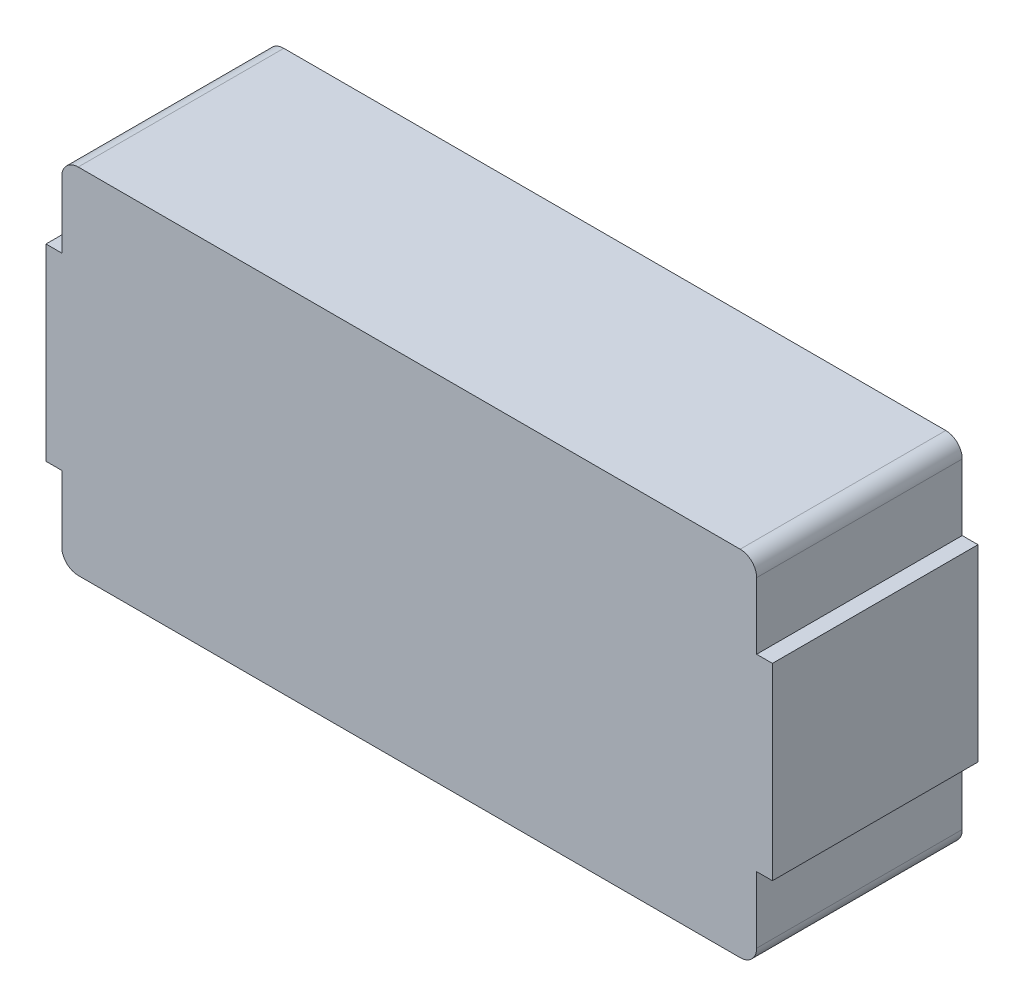
from build123d import *

# Parameters (mm, degrees)
BOSS_EXTRUDE1_DEPTH = 4
BOSS_EXTRUDE2_DEPTH = 25
FILLET1_R           = 2


with BuildPart() as part:
    # Sketch1 → Boss-Extrude1 (new body)
    with BuildSketch(Plane.XY):
        with BuildLine():
            Line((27.065651732, -12.482893197), (-27.188857752, -12.482893197))
            ThreePointArc((-27.188857752, -12.482893197), (-39.671750949, 0), (-27.188857752, 12.482893197))
            Line((-27.188857752, 12.482893197), (27.065651732, 12.482893197))
            ThreePointArc((27.065651732, 12.482893197), (39.548544929, 0), (27.065651732, -12.482893197))
        make_face()
    extrude(amount=BOSS_EXTRUDE1_DEPTH)

    # Sketch2 → Boss-Extrude2 (add)
    with BuildSketch(Plane.XY.offset(4)):
        Polygon((42.249168755, -21.510932303), (-42.249168755, -21.510932303), (-42.249168755, -11.445209118), (-44.167491565, -11.445209118), (-44.167491565, 11.445209118), (-42.249168755, 11.445209118), (-42.249168755, 21.510932303), (42.249168755, 21.510932303), (42.249168755, 11.445209118), (44.167491565, 11.445209118), (44.167491565, -11.445209118), (42.249168755, -11.445209118), align=None)
    extrude(amount=BOSS_EXTRUDE2_DEPTH)

    # Fillet1
    fillet1_edges = [part.edges().sort_by_distance(p)[0] for p in [
        (-42.249168755, 21.510932303, 16.5),
        (-42.249168755, -21.510932303, 16.5),
        (42.249168755, -21.510932303, 16.5),
        (42.249168755, 21.510932303, 16.5),
    ]]
    fillet(fillet1_edges, radius=FILLET1_R)


solid = part.part
